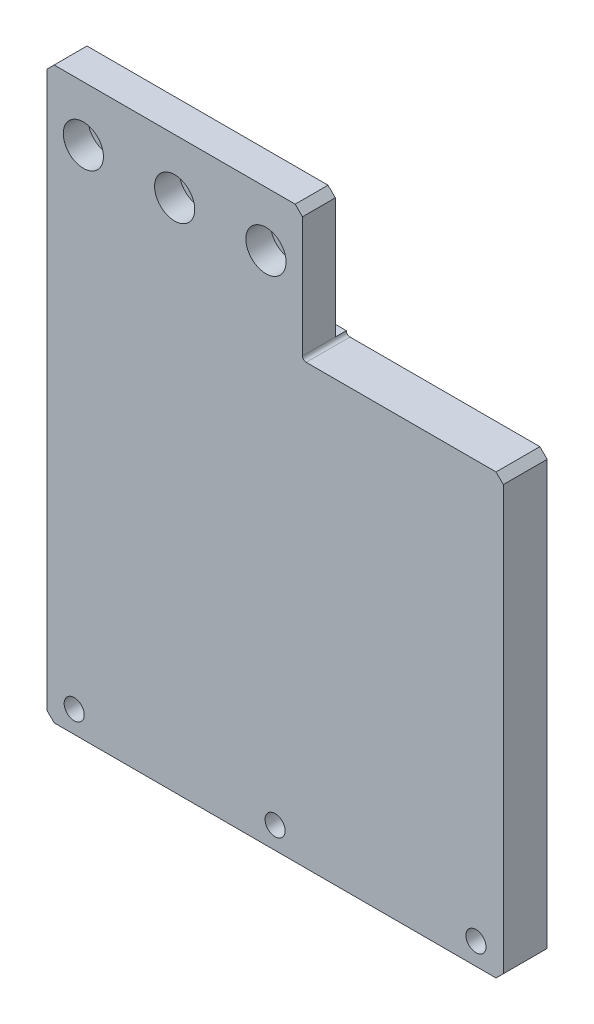
SolidWorks part; units mm, degrees
ref_plane "前视基准面" through (0, 0, 0) normal (0, 0, 1) x (1, 0, 0)
ref_plane "上视基准面" through (0, 0, 0) normal (0, 1, 0) x (1, 0, 0)
ref_plane "右视基准面" through (0, 0, 0) normal (1, 0, 0) x (0, 0, -1)
sketch "草图1" plane through (0, 0, 0) normal (0, 0, 1) x (1, 0, 0)
  line L1 (-62.5, -78) -> (62.5, -78)
  line L2 (-62.5, -78) -> (-62.5, 78)
  line L3 (-62.5, 78) -> (62.5, 78)
  line L4 (62.5, -78) -> (62.5, 78)
  line L5 (-62.5, -78) -> (62.5, 78) construction
  line L6 (-62.5, 78) -> (62.5, -78) construction
  point P0 (0, 0)
  dimension "D1" = 156
  dimension "D2" = 125
extrude "凸台-拉伸1" add sketch "草图1" along normal blind 12
sketch "草图2" plane through (0, 0, 12) normal (0, 0, 1) x (1, 0, 0)
  line L1 (62.5, 78) -> (7.5, 78)
  line L2 (62.5, 78) -> (62.5, 42)
  line L3 (62.5, 42) -> (7.5, 42)
  line L4 (7.5, 78) -> (7.5, 42)
  dimension "D1" = 55
  dimension "D2" = 36
extrude "切除-拉伸1" cut sketch "草图2" against normal through all
sketch "草图3" plane through (0, 0, 0) normal (0, 0, -1) x (-1, 0, 0)
  line L0 (-7.5, 78) -> (-7.5, 42) construction
  line L1 (62.5, 78) -> (-7.5, 78)
  line L2 (62.5, 78) -> (62.5, 43)
  line L3 (62.5, 43) -> (-7.5, 43)
  line L4 (-7.5, 78) -> (-7.5, 43)
  dimension "D1" = 35
extrude "切除-拉伸2" cut sketch "草图3" against normal blind 3
hole_wizard "打孔尺寸(%根据)内六角圆柱头螺钉的类型1" positions "草图4" profile "草图5" counterbore size "M5" standard "GB" end condition through all
sketch "草图4" plane through (0, 0, 0) normal (0, 0, -1) x (-1, 0, 0)
  line L0 (0, -78) -> (0, 0) construction
  line L1 (62.5, -78) -> (-62.5, -78) construction
  point P0 (-55, -72)
  point P2 (0, -72)
  point P4 (55, -72)
  dimension "D1" = 110
  dimension "D2" = 6
sketch "草图5" plane through (55, -72, 0) normal (1, 0, 0) x (0, 1, 0)
  line L0 (0, 0) -> (0, 12)
  line L1 (0, 12) -> (2.75, 12)
  line L3 (2.75, 12) -> (2.75, 5.7)
  line L4 (2.75, 5.7) -> (5, 5.7)
  line L5 (5, 5.7) -> (5, 0)
  line L7 (5, 0) -> (0, 0)
  line L11 (0, -6.35) -> (0, 107.95) construction
  dimension "通孔孔直径" = 5.5
  dimension "通孔孔深度" = 12
  dimension "柱形沉头孔直径" = 10
  dimension "柱形沉头孔深度" = 5.7
hole_wizard "打孔尺寸(%根据)内六角圆柱头螺钉的类型2" positions "草图6" profile "草图7" counterbore size "M6" standard "GB" end condition through all
sketch "草图6" plane through (0, 0, 12) normal (0, 0, -1) x (-1, 0, 0)
  line L0 (27.5, 78) -> (27.5, 43) construction
  line L1 (62.5, 78) -> (-7.5, 78) construction
  line L2 (-7.5, 43) -> (62.5, 43) construction
  line L4 (-7.5, 43) -> (62.5, 43) construction
  point P0 (2.5, 63)
  point P2 (27.5, 63)
  point P4 (52.5, 63)
  dimension "D1" = 50
  dimension "D2" = 20
sketch "草图7" plane through (-2.5, 63, 12) normal (1, 0, 0) x (0, -1, 0)
  line L0 (0, 0) -> (0, 12)
  line L1 (0, 12) -> (3.3, 12)
  line L3 (3.3, 12) -> (3.3, 6.8)
  line L4 (3.3, 6.8) -> (5.5, 6.8)
  line L5 (5.5, 6.8) -> (5.5, 0)
  line L7 (5.5, 0) -> (0, 0)
  line L11 (0, -6.35) -> (0, 107.95) construction
  dimension "通孔孔直径" = 6.6
  dimension "通孔孔深度" = 12
  dimension "柱形沉头孔直径" = 11
  dimension "柱形沉头孔深度" = 6.8
chamfer "倒角1" distance 2 angle 45 5 edges at (7.5, 78, 7.5) (-62.5, 78, 7.5) (62.5, 42, 6) (62.5, -78, 6) (-62.5, -78, 6)
fillet "圆角1" radius 1 1 edges at (7.5, 42, 6)
